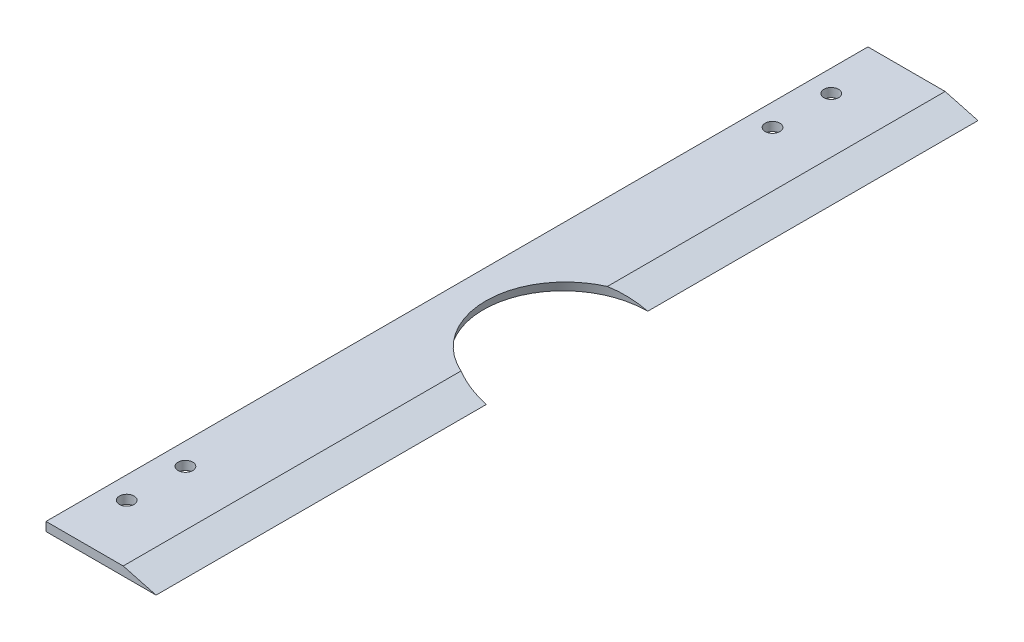
from build123d import *

# Parameters (mm, degrees)
EXTRUDE_1_DEPTH     = 280
SKETCH_2_R          = 2.5
CUT_EXTRUDE_1_DEPTH = 280
SKETCH_3_R          = 27.5
CUT_EXTRUDE_5_DEPTH = 283.433889606


with BuildPart() as part:
    # 草图1 → 凸台-拉伸1 (new body)
    with BuildSketch(Plane.XY):
        Polygon((0, 0), (0, -3), (37.5, -3), (26.303847577, 0), align=None)
    extrude(amount=EXTRUDE_1_DEPTH)

    # 草图2 → 切除-拉伸1 (cut)
    with BuildSketch(Plane(origin=(0, 0, 0), x_dir=(1, 0, 0), z_dir=(0, 1, 0))):
        with Locations(Location((7.5, -260, 0), (0, 0, 180))):
            Circle(SKETCH_2_R)
        with Locations(Location((7.5, -240, 0), (0, 0, 180))):
            Circle(SKETCH_2_R)
        with Locations(Location((7.5, -20, 0), (0, 0, 180))):
            Circle(SKETCH_2_R)
        with Locations(Location((7.5, -40, 0), (0, 0, 180))):
            Circle(SKETCH_2_R)
    extrude(amount=-CUT_EXTRUDE_1_DEPTH, mode=Mode.SUBTRACT)

    # 草图3 → 切除-拉伸5 (cut, through all)
    with BuildSketch(Plane(origin=(1.762023679, 6.575961894, 0), x_dir=(0.96592582628907, -0.2588190451025147, 0), z_dir=(0.25881904510251463, 0.9659258262890699, 0))):
        with Locations((36.998675621, -140)):
            Circle(SKETCH_3_R)
    extrude(amount=-CUT_EXTRUDE_5_DEPTH, mode=Mode.SUBTRACT)


solid = part.part
